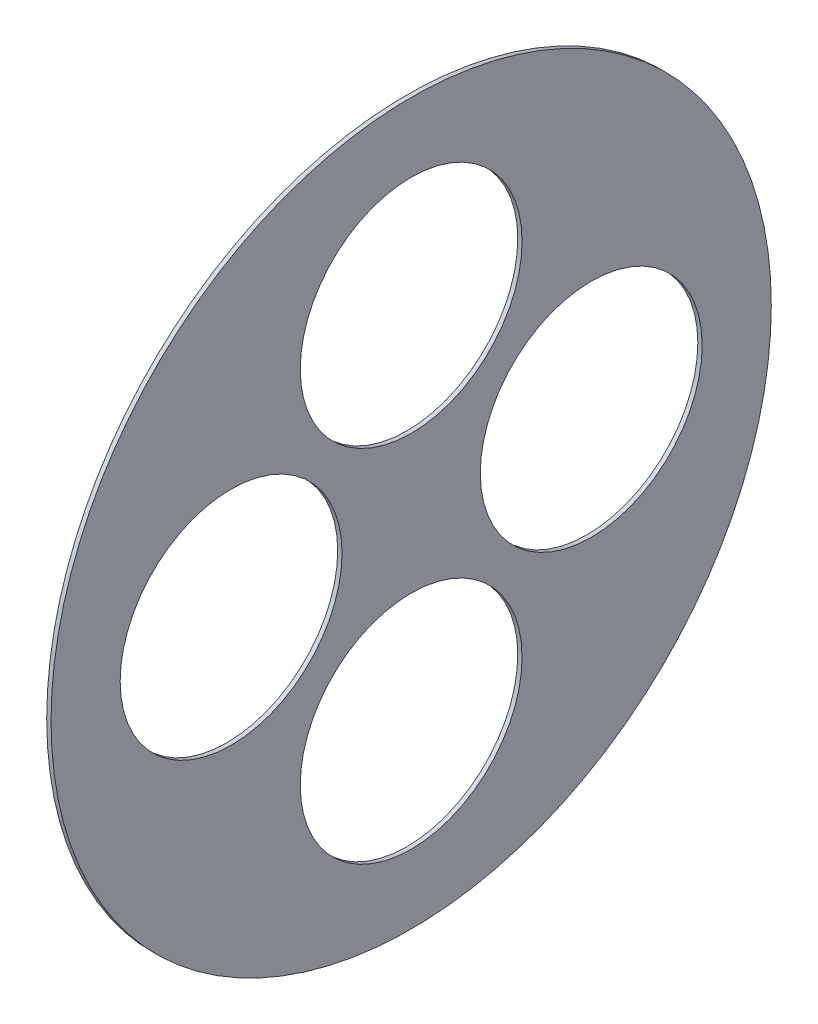
SolidWorks part; units mm, degrees
material "AISI 304"
ref_plane "Front Plane" through (0, 0, 0) normal (0, 0, 1) x (1, 0, 0)
ref_plane "Top Plane" through (0, 0, 0) normal (0, 1, 0) x (1, 0, 0)
ref_plane "Right Plane" through (0, 0, 0) normal (1, 0, 0) x (0, 0, -1)
sketch "Sketch1" plane through (0, 0, 0) normal (1, 0, 0) x (0, 0, -1)
  circle A0 centre (0, 0) radius 250
  dimension "D1" = 500
extrude "Boss-Extrude1" add sketch "Sketch1" along normal blind 3
sketch "Sketch2" plane through (3, 0, 0) normal (1, 0, 0) x (0, 0, -1)
  line L0 (0, 0) -> (0, 250) construction
  circle A0 centre (0, 125) radius 77
  dimension "D1" = 125
  dimension "D2" = 154
extrude "Cut-Extrude1" cut sketch "Sketch2" against normal blind 10
pattern_circular "CirPattern1" count 4 over 360 about axis through (0, 0, 0) along (1, 0, 0) of "Cut-Extrude1"
sketch "Sketch3" plane through (3, 0, 0) normal (1, 0, 0) x (0, 0, -1)
  line L0 (0, 0) -> (0, -312.4202) construction
  circle A0 centre (0, -237.5) radius 3
  dimension "D1" = 6
  dimension "D2" = 237.5
extrude "Cut-Extrude2" [suppressed] cut sketch "Sketch3" against normal blind 20
pattern_circular "CirPattern2" [suppressed] count 6 over 360
